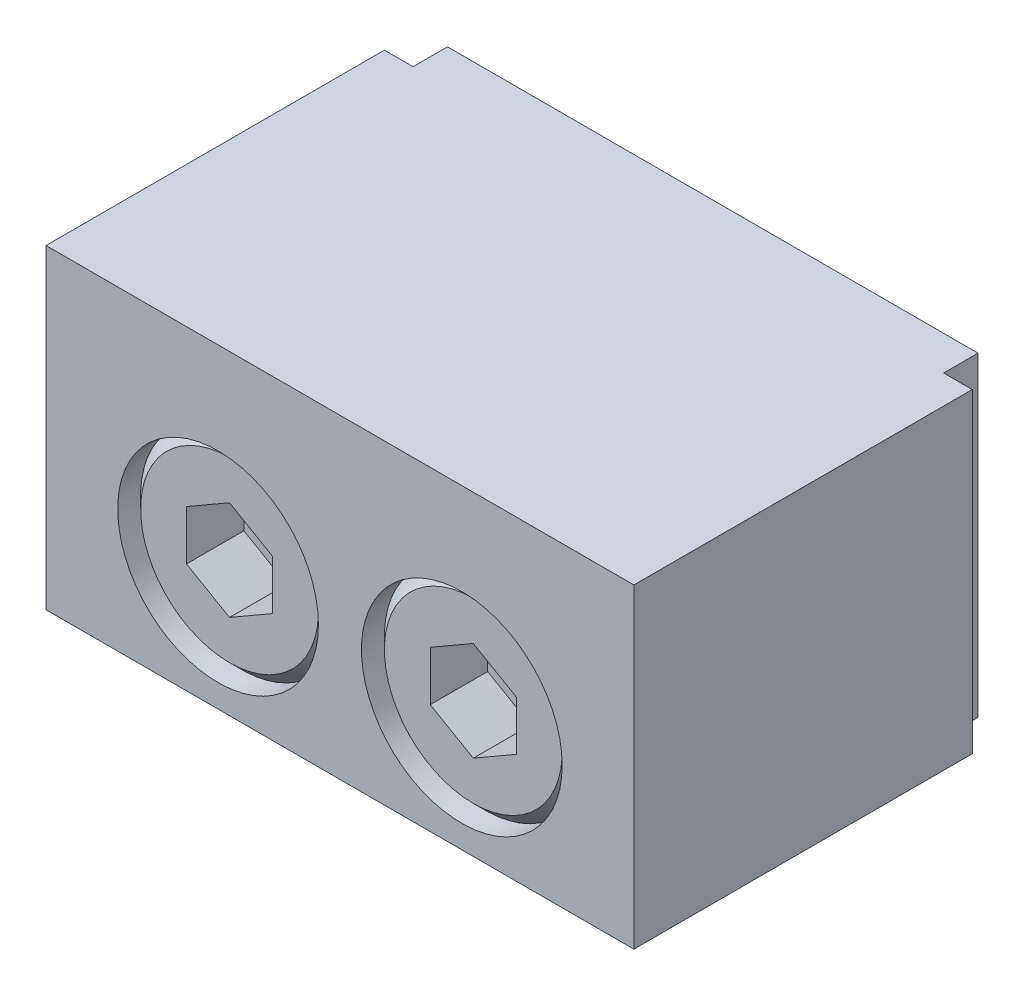
from build123d import *

# Parameters (mm, degrees)
SKETCH_1_W          = 20.5
SKETCH_1_H          = 13
EXTRUDE_1_DEPTH     = 11
CUT_EXTRUDE_1_DEPTH = 13
HOLE_WIZARD_1_D     = 7
HOLE_WIZARD_1_DEPTH = 4.4
HOLE_WIZARD_2_D     = 7
HOLE_WIZARD_2_DEPTH = 4.4
CUT_EXTRUDE_2_DEPTH = 2
CUT_EXTRUDE_3_DEPTH = 2


with BuildPart() as part:
    # 草图1 → 凸台-拉伸1 (new body)
    with BuildSketch(Plane(origin=(0, 0, 0), x_dir=(1, 0, 0), z_dir=(0, 1, 0))):
        with Locations((10.25, 6.5)):
            Rectangle(SKETCH_1_W, SKETCH_1_H)
    extrude(amount=EXTRUDE_1_DEPTH)

    # 草图2 → 切除-拉伸1 (cut)
    with BuildSketch(Plane(origin=(0, 0, 0), x_dir=(1, 0, 0), z_dir=(0, 1, 0))):
        Polygon((0, 11.8), (1, 11.8), (1, 13), (19.5, 13), (19.5, 11.8), (20.5, 11.8), (20.5, 26), (0, 26), align=None)
    extrude(amount=CUT_EXTRUDE_1_DEPTH, mode=Mode.SUBTRACT)

    # 孔1
    with Locations(Plane.XY):
        with Locations((6, 4.3)):
            Hole(HOLE_WIZARD_1_D / 2, depth=HOLE_WIZARD_1_DEPTH)

    # 孔2
    with Locations(Plane.XY):
        with Locations((14.5, 4.3)):
            Hole(HOLE_WIZARD_2_D / 2, depth=HOLE_WIZARD_2_DEPTH)

    # 草图7 → 旋转1 (revolve)
    with BuildSketch(Plane(origin=(6, 0, 0), x_dir=(0, 0, -1), z_dir=(1, 0, 0)), mode=Mode.PRIVATE) as revolve_1_sk:
        Polygon((0.4, 4.3), (0.4, 7.4), (0.8, 7.8), (4.4, 7.8), (4.4, 4.3), align=None)
    revolve(revolve_1_sk.sketch.rotate(Axis((6, 4.3, -4.4), (0, 0, 1)), 270), axis=Axis((6, 4.3, -4.4), (0, 0, 1)))

    # 草图8 → 旋转2 (revolve)
    with BuildSketch(Plane(origin=(14.5, 0, 0), x_dir=(0, 0, -1), z_dir=(1, 0, 0)), mode=Mode.PRIVATE) as revolve_2_sk:
        Polygon((0.4, 4.3), (0.4, 7.4), (0.8, 7.8), (4.4, 7.8), (4.4, 4.3), align=None)
    revolve(revolve_2_sk.sketch.rotate(Axis((14.5, 4.3, -4.4), (0, 0, 1)), 270), axis=Axis((14.5, 4.3, -4.4), (0, 0, 1)))

    # 草图9 → 切除-拉伸2 (cut)
    with BuildSketch(Plane.XY.offset(-0.4)):
        Polygon((4.5, 5.166025404), (4.5, 3.433974596), (6, 2.567949192), (7.5, 3.433974596), (7.5, 5.166025404), (6, 6.032050808), align=None)
    extrude(amount=-CUT_EXTRUDE_2_DEPTH, mode=Mode.SUBTRACT)

    # 草图10 → 切除-拉伸3 (cut)
    with BuildSketch(Plane.XY.offset(-0.4)):
        Polygon((13, 3.433974596), (14.5, 2.567949192), (16, 3.433974596), (16, 5.166025404), (14.5, 6.032050808), (13, 5.166025404), align=None)
    extrude(amount=-CUT_EXTRUDE_3_DEPTH, mode=Mode.SUBTRACT)


solid = part.part
